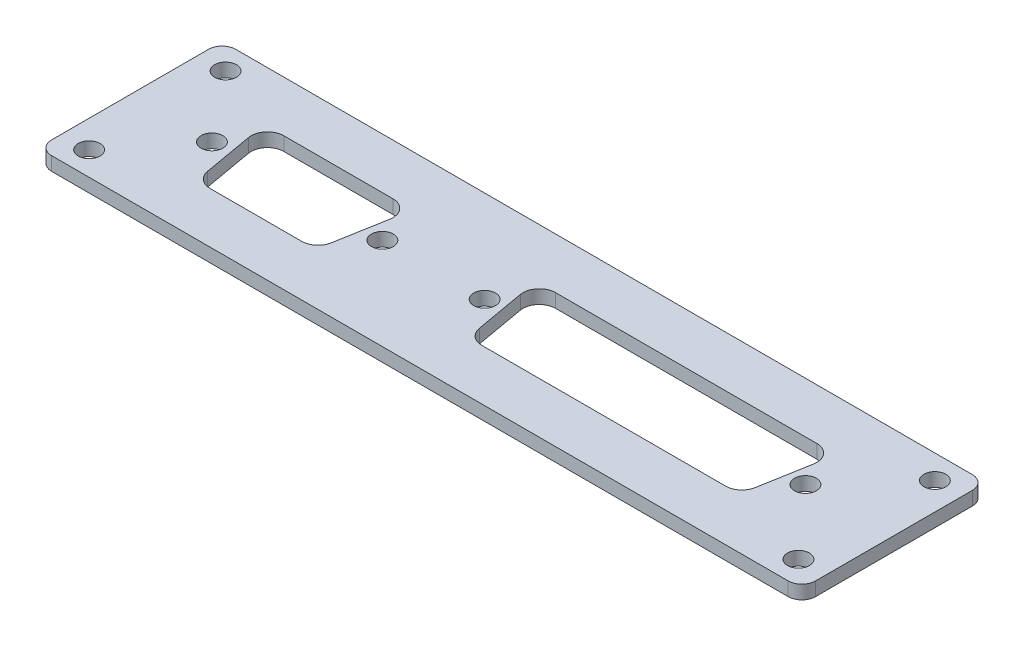
SolidWorks part; units mm, degrees
ref_plane "Front Plane" through (0, 0, 0) normal (0, 0, 1) x (1, 0, 0)
ref_plane "Top Plane" through (0, 0, 0) normal (0, 1, 0) x (1, 0, 0)
ref_plane "Right Plane" through (0, 0, 0) normal (1, 0, 0) x (0, 0, -1)
sketch "Sketch1" plane through (0, 0, 0) normal (0, 1, 0) x (1, 0, 0)
  line L1 (-56, -13.5) -> (56, -13.5)
  line L2 (-56, -13.5) -> (-56, 13.5)
  line L3 (-56, 13.5) -> (56, 13.5)
  line L4 (56, -13.5) -> (56, 13.5)
  line L5 (-56, -13.5) -> (56, 13.5) construction
  line L6 (-56, 13.5) -> (56, -13.5) construction
  point P0 (0, 0)
  dimension "D1" = 112
  dimension "D2" = 27
extrude "Boss-Extrude1" add sketch "Sketch1" along normal blind 2
sketch "Sketch2" plane through (0, 2, 0) normal (0, 1, 0) x (1, 0, 0)
  line L1 (-52, -10) -> (52, -10) construction
  line L2 (-52, -10) -> (-52, 10) construction
  line L3 (-52, 10) -> (52, 10) construction
  line L4 (52, -10) -> (52, 10) construction
  line L5 (-52, -10) -> (52, 10) construction
  line L6 (-52, 10) -> (52, -10) construction
  circle A0 centre (-52, 10) radius 1.6
  circle A1 centre (52, 10) radius 1.6
  circle A2 centre (52, -10) radius 1.6
  circle A3 centre (-52, -10) radius 1.6
  point P0 (0, 0)
  dimension "D3" = 3.2
  dimension "D4" = 3.2
  dimension "D5" = 3.2
  dimension "D6" = 3.2
  dimension "D1" = 20
  dimension "D2" = 104
extrude "Cut-Extrude1" cut sketch "Sketch2" against normal through all
fillet "Fillet1" radius 2 4 edges at (56, 1, -13.5) (56, 1, 13.5) (-56, 1, 13.5) (-56, 1, -13.5)
sketch "Sketch3" plane through (0, 2, 0) normal (0, 1, 0) x (1, 0, 0)
  line L8 (-39.5, 5.75) -> (-23.5, 5.75) construction
  line L9 (-21.4319, 3.2853) -> (-22.7191, -4.0147) construction
  line L10 (-24.7872, -5.75) -> (-38.2128, -5.75) construction
  line L11 (-40.2809, -4.0147) -> (-41.5681, 3.2853) construction
  line L12 (0.35, 5.75) -> (38.65, 5.75) construction
  line L13 (40.7181, 3.2853) -> (39.4309, -4.0147) construction
  line L14 (37.3628, -5.75) -> (1.6372, -5.75) construction
  line L15 (-0.4309, -4.0147) -> (-1.7181, 3.2853) construction
  line L16 (41.1527, 5.75) -> (41.1527, 7.5) construction
  line L17 (-2.1527, 5.75) -> (-2.1527, 8.0893) construction
  line L18 (-20.9973, 5.75) -> (-20.9973, 8.0893) construction
  line L19 (-42.0027, 5.75) -> (-42.0027, 8.0893) construction
  line L20 (37.3628, -6.05) -> (1.6372, -6.05)
  line L21 (-0.7264, -4.0668) -> (-2.0135, 3.2332)
  line L22 (0.35, 6.05) -> (38.65, 6.05)
  line L23 (41.0135, 3.2332) -> (39.7264, -4.0668)
  line L24 (-39.5, 6.05) -> (-23.5, 6.05)
  line L25 (-21.1365, 3.2332) -> (-22.4236, -4.0668)
  line L26 (-24.7872, -6.05) -> (-38.2128, -6.05)
  line L27 (-40.5764, -4.0668) -> (-41.8635, 3.2332)
  arc A0 (-23.5, 5.75) -> (-21.4319, 3.2853) centre (-23.5, 3.65) cw construction
  arc A1 (-39.5, 5.75) -> (-41.5681, 3.2853) centre (-39.5, 3.65) ccw construction
  arc A2 (-38.2128, -5.75) -> (-40.2809, -4.0147) centre (-38.2128, -3.65) cw construction
  arc A3 (-22.7191, -4.0147) -> (-24.7872, -5.75) centre (-24.7872, -3.65) cw construction
  arc A4 (1.6372, -5.75) -> (-0.4309, -4.0147) centre (1.6372, -3.65) cw
  arc A5 (0.35, 5.75) -> (-1.7181, 3.2853) centre (0.35, 3.65) ccw construction
  arc A6 (38.65, 5.75) -> (40.7181, 3.2853) centre (38.65, 3.65) cw construction
  arc A7 (39.4309, -4.0147) -> (37.3628, -5.75) centre (37.3628, -3.65) cw construction
  circle A8 centre (-43.995, 0) radius 1.6
  circle A9 centre (-19.005, 0) radius 1.6
  circle A10 centre (-4.02, 0) radius 1.6
  circle A11 centre (43.02, 0) radius 1.6
  arc A12 (1.6372, -6.05) -> (-0.7264, -4.0668) centre (1.6372, -3.65) cw
  arc A13 (0.35, 6.05) -> (-2.0135, 3.2332) centre (0.35, 3.65) ccw
  arc A14 (38.65, 6.05) -> (41.0135, 3.2332) centre (38.65, 3.65) cw
  arc A15 (39.7264, -4.0668) -> (37.3628, -6.05) centre (37.3628, -3.65) cw
  arc A16 (-23.5, 6.05) -> (-21.1365, 3.2332) centre (-23.5, 3.65) cw
  arc A17 (-22.4236, -4.0668) -> (-24.7872, -6.05) centre (-24.7872, -3.65) cw
  arc A18 (-38.2128, -6.05) -> (-40.5764, -4.0668) centre (-38.2128, -3.65) cw
  arc A19 (-39.5, 6.05) -> (-41.8635, 3.2332) centre (-39.5, 3.65) ccw
  point P50 (-31.5, 5.75)
  point P51 (19.5, 5.75)
  dimension "D5" = 2.1
  dimension "D13" = 3.2
  dimension "D15" = 3.2
  dimension "D16" = 23.52
  dimension "D18" = 3.2
  dimension "D21" = 3.2
  dimension "D1" = 10
  dimension "D2" = 10
  dimension "D3" = 10
  dimension "D4" = 10
  dimension "D6" = 38.3
  dimension "D7" = 16
  dimension "D8" = 11.5
  dimension "D9" = 11.5
  dimension "D10" = 5.75
  dimension "D14" = 23.52
  dimension "D17" = 180
  dimension "D19" = 12.495
  dimension "D20" = 12.495
  dimension "D22" = 0.3
  dimension "D23" = 0.3
extrude "Cut-Extrude2" cut sketch "Sketch3" against normal blind 2
